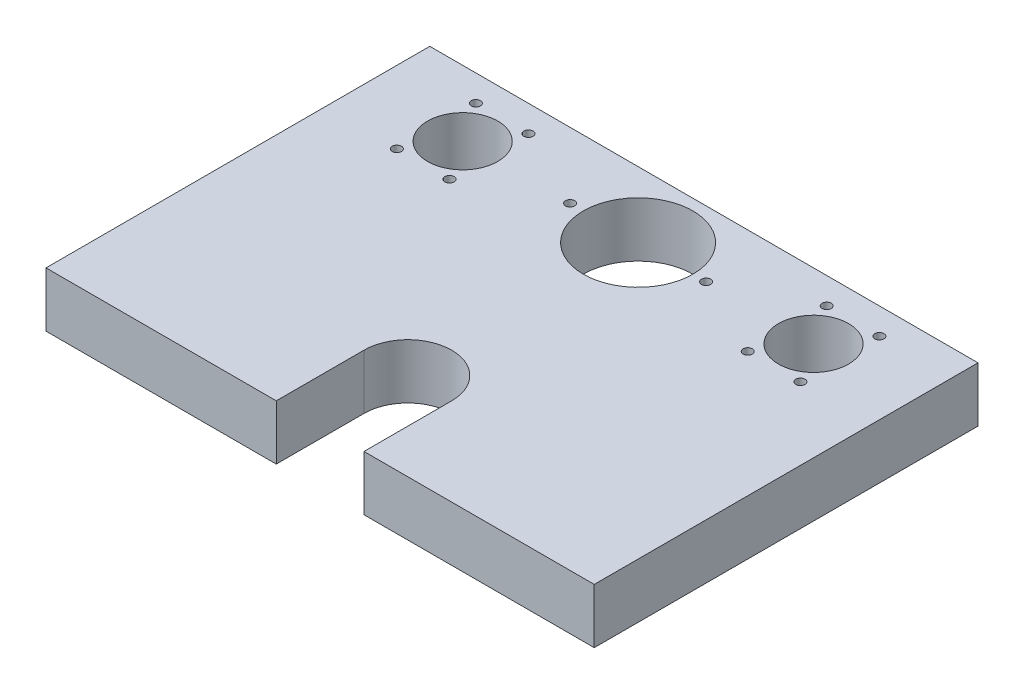
from build123d import *

# Parameters (mm, degrees)
SKETCH1_W                  = 250
SKETCH1_H                  = 175
BOSS_EXTRUDE1_DEPTH        = 25
CUT_EXTRUDE1_DEPTH         = 155.616460961
SKETCH3_R                  = 16
CUT_EXTRUDE2_DEPTH         = 155.616460961
M5_TAPPED_HOLE2_AT_2_COUNT = 2
M5_TAPPED_HOLE2_AT_2_PITCH = 24
M5_TAPPED_HOLE2_AT_3_COUNT = 2
M5_TAPPED_HOLE2_AT_3_PITCH = 36
M5_TAPPED_HOLE2_AT_4_COUNT = 2
M5_TAPPED_HOLE2_AT_4_PITCH = 43.266615306
SKETCH7_R                  = 25
CUT_EXTRUDE3_DEPTH         = 155.616460961
M5_TAPPED_HOLE1_D          = 4.2


with BuildPart() as part:
    # Sketch1 → Boss-Extrude1 (new body)
    with BuildSketch(Plane(origin=(0, 0, 0), x_dir=(1, 0, 0), z_dir=(0, 1, 0))):
        Rectangle(SKETCH1_W, SKETCH1_H)
    extrude(amount=BOSS_EXTRUDE1_DEPTH)

    # Sketch2 → Cut-Extrude1 (cut, through all)
    with BuildSketch(Plane(origin=(0, 25, 0), x_dir=(1, 0, 0), z_dir=(0, 1, 0))):
        with BuildLine():
            Line((-20, -47.5), (-20, -87.5))
            Line((-20, -87.5), (20, -87.5))
            Line((20, -87.5), (20, -47.5))
            ThreePointArc((20, -47.5), (0, -27.5), (-20, -47.5))
        make_face()
    extrude(amount=-CUT_EXTRUDE1_DEPTH, mode=Mode.SUBTRACT)

    # Sketch3 → Cut-Extrude2 (cut, through all)
    with BuildSketch(Plane(origin=(0, 25, 0), x_dir=(1, 0, 0), z_dir=(0, 1, 0))):
        with Locations(Location((-80, 57.5, 0), (0, 0, 270))):
            Circle(SKETCH3_R)
        with Locations(Location((80, 57.5, 0), (0, 0, 90))):
            Circle(SKETCH3_R)
    extrude(amount=-CUT_EXTRUDE2_DEPTH, mode=Mode.SUBTRACT)

    # Sketch6 → M5 Tapped Hole2 (revolve, cut)
    with BuildSketch(Plane(origin=(-92, 25, -75.5), x_dir=(0, 0, 1), z_dir=(1, 0, 0))):
        Polygon((0, 0), (0, 13.6618073), (2.1, 12.4), (2.1, 0), align=None)
    m5_tapped_hole2 = revolve(axis=Axis((-92, 31.35, -75.5), (0, -1, 0)), mode=Mode.SUBTRACT)

    # M5 Tapped Hole2 at 2: M5 Tapped Hole2 ×2
    with Locations(*[(i * M5_TAPPED_HOLE2_AT_2_PITCH, 0, 0) for i in range(1, M5_TAPPED_HOLE2_AT_2_COUNT)]):
        add(m5_tapped_hole2, mode=Mode.SUBTRACT)

    # M5 Tapped Hole2 at 3: M5 Tapped Hole2 ×2
    with Locations(*[(0, 0, i * M5_TAPPED_HOLE2_AT_3_PITCH) for i in range(1, M5_TAPPED_HOLE2_AT_3_COUNT)]):
        add(m5_tapped_hole2, mode=Mode.SUBTRACT)

    # M5 Tapped Hole2 at 4: M5 Tapped Hole2 ×2
    with Locations(*[Vector(0.5547001962252294, 0, 0.8320502943378435) * (i * M5_TAPPED_HOLE2_AT_4_PITCH) for i in range(1, M5_TAPPED_HOLE2_AT_4_COUNT)]):
        add(m5_tapped_hole2, mode=Mode.SUBTRACT)

    # Mirror1: M5 Tapped Hole2 across plane
    add(m5_tapped_hole2.mirror(Plane(origin=(0, 0, 0), x_dir=(0, 0, 1), z_dir=(1, 0, 0))), mode=Mode.SUBTRACT)

    # Mirror1 copy 1 sketch → Mirror1 copy 1 (revolve, cut)
    with BuildSketch(Plane(origin=(68, 25, -75.5), x_dir=(0, 0, 1), z_dir=(-1, 0, 0))):
        Polygon((0, 0), (0, -13.6618073), (2.1, -12.4), (2.1, 0), align=None)
    revolve(axis=Axis((68, 31.35, -75.5), (0, 1, 0)), mode=Mode.SUBTRACT)

    # Mirror1 copy 2 sketch → Mirror1 copy 2 (revolve, cut)
    with BuildSketch(Plane(origin=(92, 25, -39.5), x_dir=(0, 0, 1), z_dir=(-1, 0, 0))):
        Polygon((0, 0), (0, -13.6618073), (2.1, -12.4), (2.1, 0), align=None)
    revolve(axis=Axis((92, 31.35, -39.5), (0, 1, 0)), mode=Mode.SUBTRACT)

    # Mirror1 copy 3 sketch → Mirror1 copy 3 (revolve, cut)
    with BuildSketch(Plane(origin=(68, 25, -39.5), x_dir=(0, 0, 1), z_dir=(-1, 0, 0))):
        Polygon((0, 0), (0, -13.6618073), (2.1, -12.4), (2.1, 0), align=None)
    revolve(axis=Axis((68, 31.35, -39.5), (0, 1, 0)), mode=Mode.SUBTRACT)

    # Sketch7 → Cut-Extrude3 (cut, through all)
    with BuildSketch(Plane(origin=(0, 25, 0), x_dir=(1, 0, 0), z_dir=(0, 1, 0))):
        with Locations(Location((0, 57.5, 0), (0, 0, 270))):
            Circle(SKETCH7_R)
    extrude(amount=-CUT_EXTRUDE3_DEPTH, mode=Mode.SUBTRACT)

    # M5 Tapped Hole1 (through all)
    with Locations(Plane(origin=(0, 25, 0), x_dir=(1, 0, 0), z_dir=(0, 1, 0))):
        with Locations((-31, 57.5), (31, 57.5)):
            Hole(M5_TAPPED_HOLE1_D / 2)


solid = part.part
